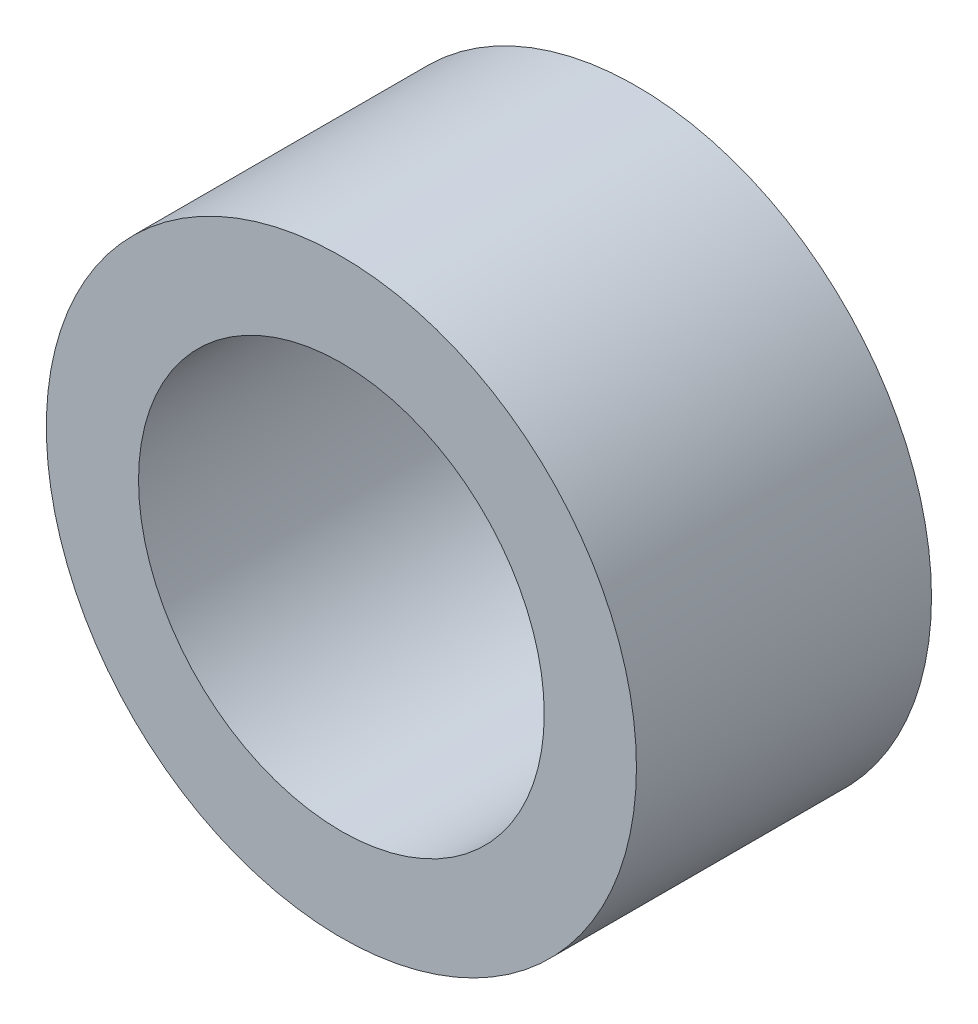
from build123d import *

# Parameters (mm, degrees)
SKETCH_1_R      = 12
SKETCH_1_R_2    = 8.25
EXTRUDE_1_DEPTH = 12


with BuildPart() as part:
    # 草图1 → 凸台-拉伸1 (new body)
    with BuildSketch(Plane.XY):
        Circle(SKETCH_1_R)
        Circle(SKETCH_1_R_2, mode=Mode.SUBTRACT)
    extrude(amount=EXTRUDE_1_DEPTH)


solid = part.part
